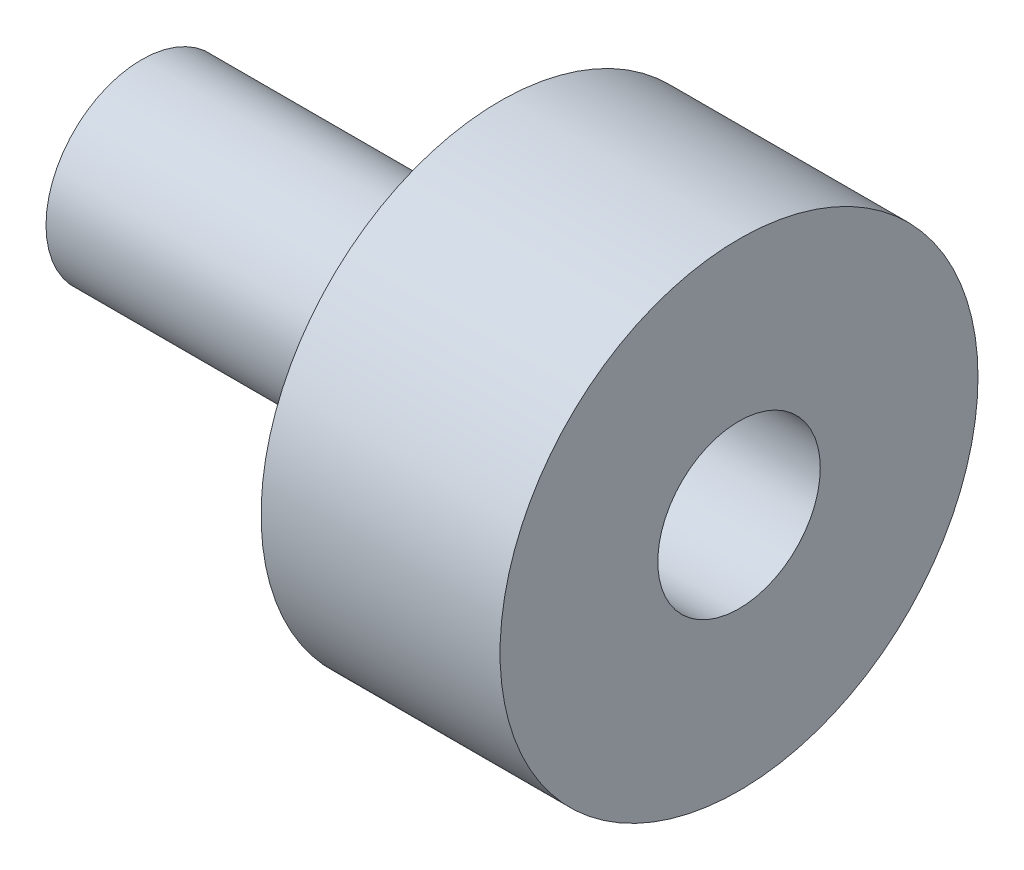
SolidWorks part; units mm, degrees
ref_plane "前视基准面" through (0, 0, 0) normal (0, 0, 1) x (1, 0, 0)
ref_plane "上视基准面" through (0, 0, 0) normal (0, 1, 0) x (1, 0, 0)
ref_plane "右视基准面" through (0, 0, 0) normal (1, 0, 0) x (0, 0, -1)
sketch "草图1" plane through (0, 0, 0) normal (1, 0, 0) x (0, 0, -1)
  circle A0 centre (0, 0) radius 10
  dimension "D1" = 20
extrude "凸台-拉伸1" add sketch "草图1" along normal blind 10 contours A0
sketch "草图2" plane through (0, 0, 0) normal (-1, 0, 0) x (0, 0, 1)
  circle A0 centre (0, 0) radius 4
  dimension "D1" = 8
extrude "凸台-拉伸2" add sketch "草图2" along normal blind 15
cosmetic thread "装饰螺纹线1" parameters "D2"=7
hole_wizard "M8 螺纹孔1" positions "草图3" profile "草图4" tap size "M8" standard "ISO"
sketch "草图3" plane through (10, 0, 0) normal (1, 0, 0) x (0, 0, -1)
  point P0 (0, 0)
sketch "草图4" plane through (10, 0, 0) normal (0, 1, 0) x (0, 0, -1)
  line L0 (0, 0) -> (0, 10.0429)
  line L1 (0, 10.0429) -> (3.4, 8)
  line L2 (3.4, 8) -> (3.4, 0)
  line L5 (3.4, 0) -> (0, 0)
  line L10 (0, 10.0429) -> (-3.4, 8) construction
  line L11 (0, -6.35) -> (0, 107.95) construction
  dimension "螺纹孔钻头直径" = 6.8
  dimension "螺纹孔钻头深度" = 8
  dimension "导头角度" = 118
cosmetic thread "孔螺蚊线1" parameters "D1"=8, "D2"=8
